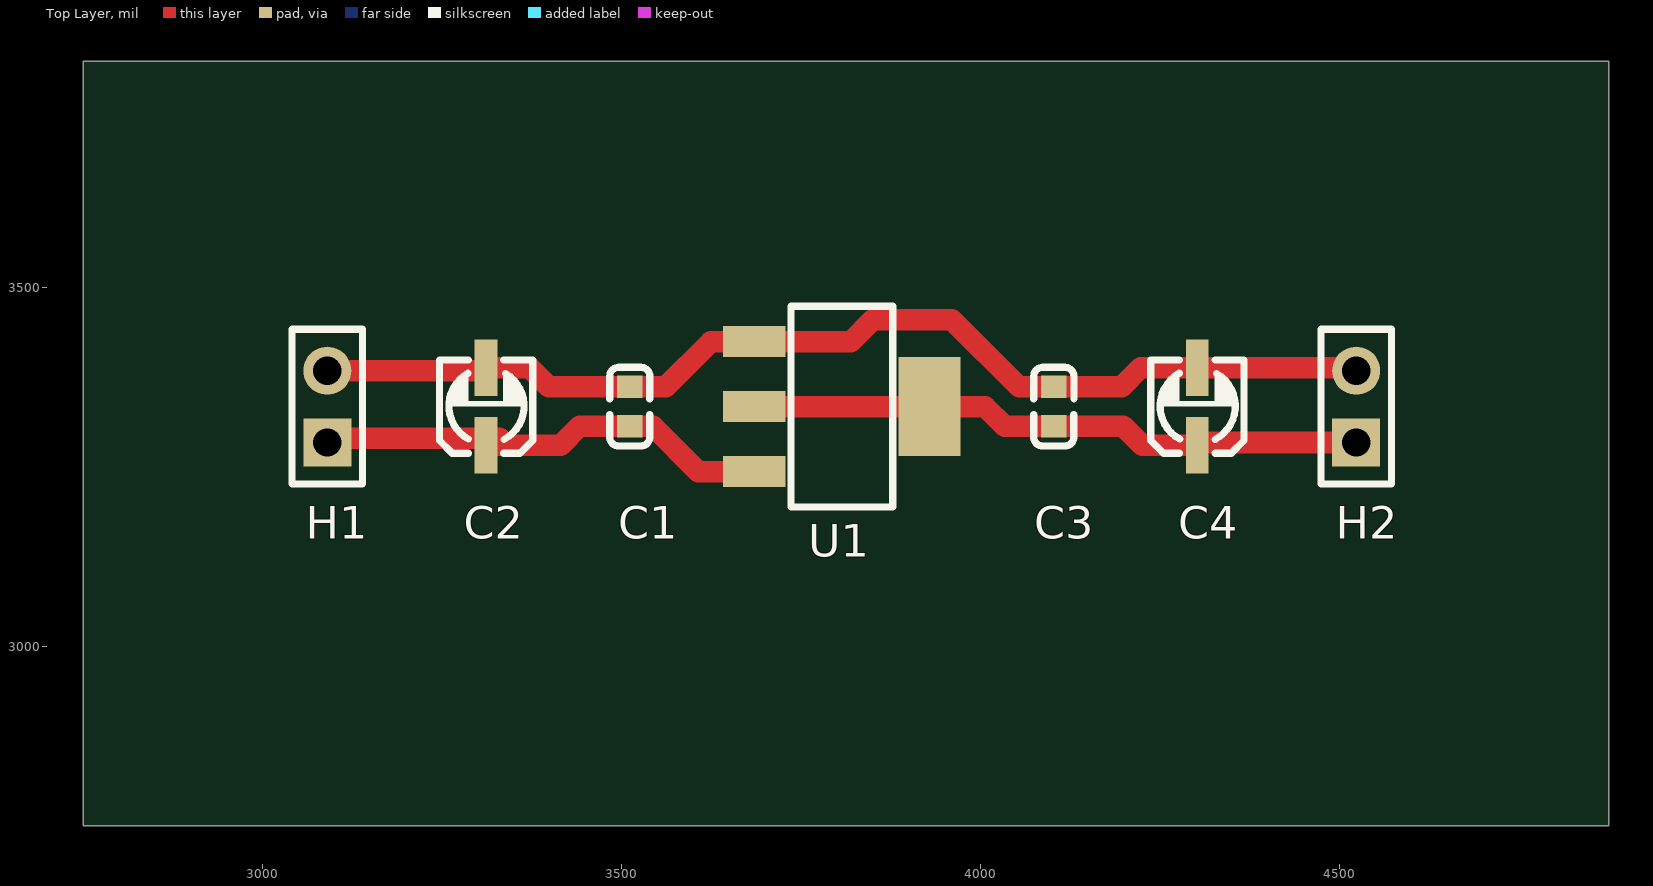
[diagram p0: Top Layer view]
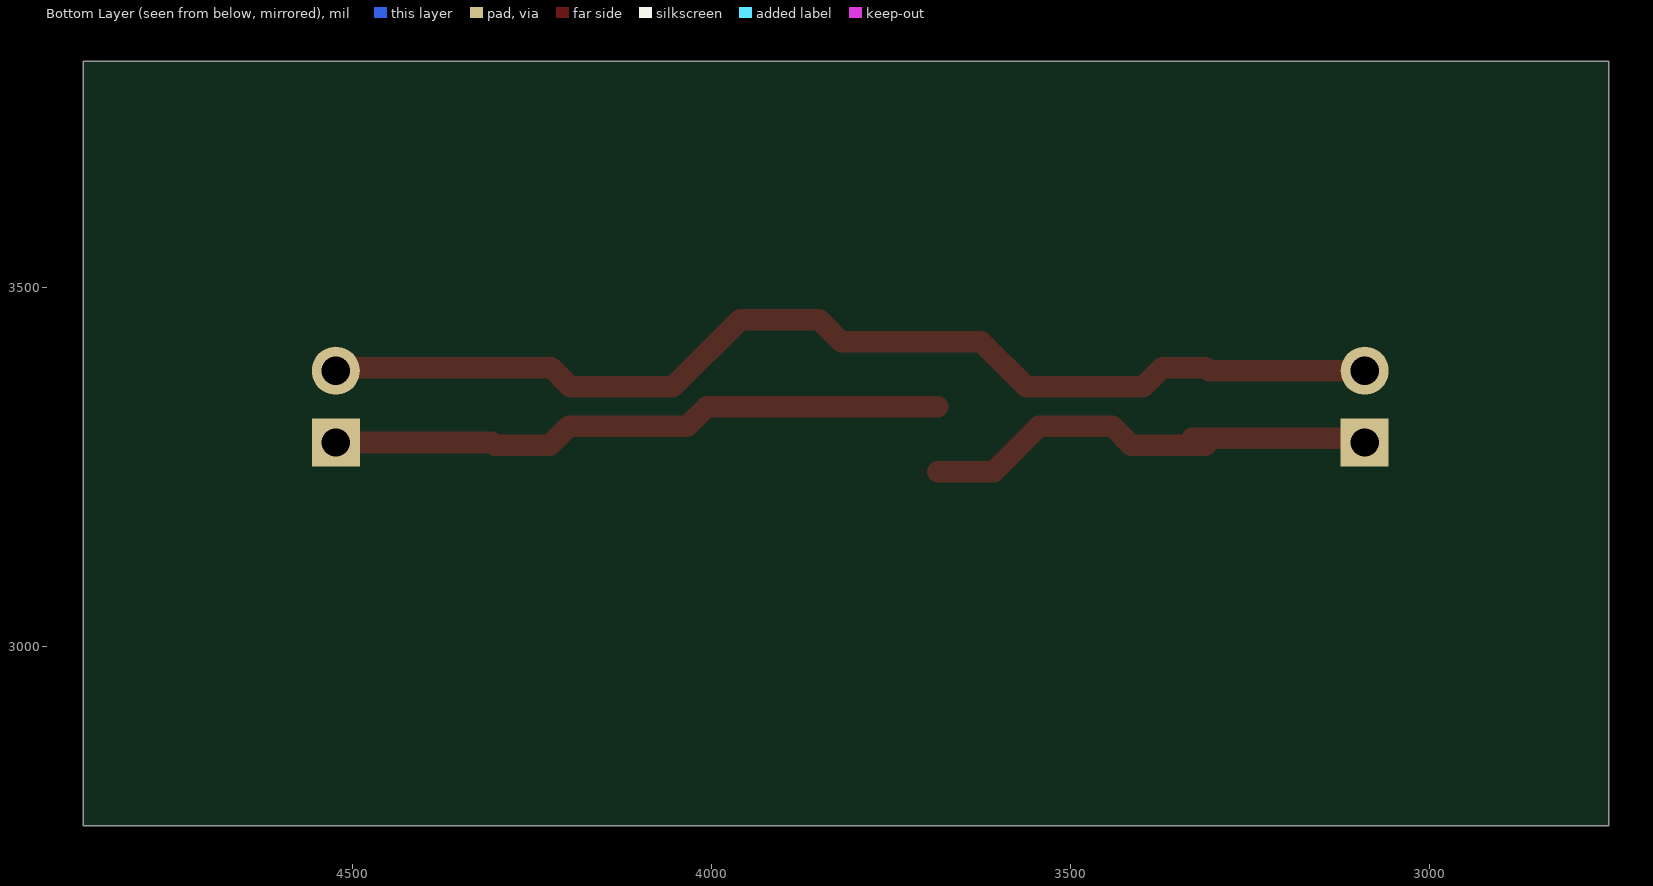
[diagram p1: Bottom Layer view, seen from below]
# Altium PCB MISC52016.pcbdoc
Units mil, origin at the board's own origin, x right, y up, seen from the top; angles counter-clockwise.
Board outline 2125 x 1065 mil, 2 copper layers (Top Layer, Bottom Layer), stack 62.206 mil thick; 7 components, 3 nets, 16 pads, 0 vias.

## Layer stack, top to bottom
Top Solder Mask Layer: solder mask 0.394, Dk 3.3
Top Layer: signal copper 1.379
Dielectric1: surface 59.449, FR4, Dk 4.5
Bottom Layer: signal copper 1.378
Bottom Solder Mask Layer: solder mask 0.394, Dk 3.3

## Board outline
4875,2750 2750,2750 2750,3815 4875,3815

## Design rules (kind name [scope] priority, off if disabled: settings)
BoardOutlineClearance copperThickness2oz_1 [All] p2 off: genericclearance=7.99 ignorepadtopadclearanceinfootprint=FALSE except(0: Arc-SplitContinuation Track-SplitContinuation SMDPad-SplitContinuation THPad-SplitContinuation Via-SplitContinuation Fill-SplitContinuation Region-SplitContinuation Poly-SplitContinuation Text-SplitContinuation Hole-SplitContinuation; 5.98: Arc-CutoutEdge SMDPad-CutoutEdge THPad-CutoutEdge Via-CutoutEdge Fill-CutoutEdge Region-CutoutEdge Text-CutoutEdge; 6.93: Hole-OutlineEdge Hole-CutoutEdge; 10: Poly-OutlineEdge Poly-CutoutEdge; 11.81: Arc-OutlineEdge Track-OutlineEdge SMDPad-OutlineEdge THPad-OutlineEdge Via-OutlineEdge Fill-OutlineEdge Region-OutlineEdge Text-OutlineEdge Track-CutoutEdge)
BoardOutlineClearance copperThickness1oz_1 [All] p4: genericclearance=4.02 ignorepadtopadclearanceinfootprint=FALSE except(0: Arc-SplitContinuation Track-SplitContinuation SMDPad-SplitContinuation THPad-SplitContinuation Via-SplitContinuation Fill-SplitContinuation Region-SplitContinuation Poly-SplitContinuation Text-SplitContinuation Hole-SplitContinuation; 6: SMDPad-CutoutEdge THPad-CutoutEdge Via-CutoutEdge Fill-CutoutEdge Region-CutoutEdge Text-CutoutEdge; 6.93: Hole-OutlineEdge Hole-CutoutEdge; 10: Poly-OutlineEdge Poly-CutoutEdge; 11.8: Arc-OutlineEdge Track-OutlineEdge SMDPad-OutlineEdge THPad-OutlineEdge Via-OutlineEdge Fill-OutlineEdge Region-OutlineEdge Text-OutlineEdge; 11.81: Arc-CutoutEdge Track-CutoutEdge)
Clearance copperThickness2oz [All] p1 off: gap=7.99 ignorepadtopadclearanceinfootprint=FALSE except(5.98: SMDPad-Track SMDPad-SMDPad THPad-Track SMDPad-THPad THPad-THPad Track-Via SMDPad-Via THPad-Via Via-Via Fill-Track Region-Track Fill-SMDPad Region-SMDPad Fill-THPad Region-THPad Fill-Via Region-Via Fill-Fill Fill-Region Region-Region Arc-Track Arc-SMDPad Arc-THPad Arc-Via Fill-Arc Region-Arc Arc-Arc Text-Track SMDPad-Text Text-THPad Text-Via Fill-Text Region-Text Arc-Text Text-Text; 6.93: Hole-Track Hole-SMDPad Hole-THPad Hole-Via Fill-Hole Region-Hole Hole-Arc Hole-Text; 10: Poly-Track Poly-SMDPad Poly-THPad Poly-Via Poly-Fill Poly-Region Poly-Poly Poly-Arc Poly-Text Poly-Hole)
Clearance copperThickness1oz [All] p3: gap=4.02 ignorepadtopadclearanceinfootprint=FALSE except(5.98: SMDPad-Track SMDPad-SMDPad THPad-Track SMDPad-THPad THPad-THPad Track-Via SMDPad-Via THPad-Via Via-Via Fill-Track Region-Track Fill-SMDPad Region-SMDPad Fill-THPad Region-THPad Fill-Via Region-Via Fill-Fill Fill-Region Region-Region; 6: Arc-Track Arc-SMDPad Arc-THPad Arc-Via Fill-Arc Region-Arc Arc-Arc Text-Track SMDPad-Text Text-THPad Text-Via Fill-Text Region-Text Arc-Text Text-Text; 6.93: Hole-Track Hole-SMDPad Hole-THPad Hole-Via Fill-Hole Region-Hole Hole-Arc Hole-Text; 10: Poly-Track Poly-SMDPad Poly-THPad Poly-Via Poly-Fill Poly-Region Poly-Poly Poly-Arc Poly-Text Poly-Hole)
DiffPairsRouting differentialPair [All] p1: maxlimit=6 minlimit=6 mostfreqgap=6 toplayer_minwidth=5 toplayer_prefwidth=10 toplayer_maxwidth=100 toplayer_mingap=6 toplayer_prefgap=6 toplayer_maxgap=6 bottomlayer_minwidth=5 bottomlayer_prefwidth=10 bottomlayer_maxwidth=100 bottomlayer_mingap=6 bottomlayer_prefgap=6 bottomlayer_maxgap=6 maxuncoupledlength=10
HoleToHoleClearance otherClearance [All] p1: gap=11.81 allowstackedmicrovias=TRUE
Length netLength [All] p1: minlimit=0 maxlimit=0
MatchedLengths netLengthTolerance [All] p1: tolerance=1000
PasteMaskExpansion pasteMaskExpansion [All] p1: expansion=0
PlaneConnect innerPlane [All] p1: planeconnectstyle=Relief reliefexpansion=20 reliefentries=4 reliefconductorwidth=10 reliefairgap=10
PolygonConnect copperRegion [All] p1: connectstyle=Relief reliefconductorwidth=10 reliefentries=4 polygonreliefangle="90 Angle" airgapwidth=10 via.connectstyle=Relief via.reliefconductorwidth=10 via.reliefentries=4 via.polygonreliefangle="90 Angle" via.airgapwidth=10
RoutingVias viaSize [All] p1: holewidth=12.01 width=24.02 viastyle="Through Hole" minholewidth=11.81 minwidth=19.68 maxholewidth=248.03 maxwidth=393.7
SolderMaskExpansion solderMaskExpansion [IsVia] p1: expansion=-1000 istentingtop=TRUE
SolderMaskExpansion solderMaskExpansion [All] p2: expansion=2 istentingtop=FALSE
Width copperThickness2oz_2 [All] p1 off: maxlimit=100 minlimit=8 preferedwidth=10
Width copperThickness1oz_2 [All] p2: maxlimit=100 minlimit=5 preferedwidth=10

## Components (designator, comment, footprint, x,y, rotation, side; value= is the part's Value field where it differs from the comment)
C1 "100nF" C0603 3511.29,3333.9 r270 top
C2 "10uF" C_Ele_SMD_3x5.4mm 3311.63,3334.1 r270 top
C3 "100nF" C0603 4101.93,3333.9 r270 top
C4 "10uF" C_Ele_SMD_3x5.4mm 4302.3,3334.1 r270 top
H1 "" HDR-TH_2P-P2.54-V-F 3090,3333.9 r90 top
H2 "" HDR-TH_2P-P2.54-V-F 4523.22,3333.9 r90 top
U1 "" SOT_223 3807.67,3333.9 r270 top

## Footprints (in the part's own frame and the unit in brackets; to place one, negate y for a bottom-side part, rotate by r counter-clockwise, add the part's x,y. Pads: shape width x height; smd on the part's side, far side on the other; paste and mask are expansions set on the pad)
C0603 [mm]
  rect 0.8x0.9 smd: 1(-0.7,0) 2(0.7,0)
  silkscreen extent -1.39,-0.71 1.39,0.71
C_Ele_SMD_3x5.4mm [mil]
  rect 78.7x31.5 smd paste+0 mask+2: 1(54.1,-0.55) 2(-53.7,-0.55)
  silkscreen extent -65,-65 65,65
HDR-TH_2P-P2.54-V-F [mm]
  rect 1.7x1.7 hole 1: 1(-1.27,0)
  round 1.7 hole 1: 2(1.27,0)
  silkscreen extent -2.74,-1.25 2.74,1.25
SOT_223 [mil]
  rect 43.3x86.6 smd paste+0 mask+2: 1(-90.5,-123.05) 2(0,-123.05) 3(90.6,-123.05)
  rect 137.8x86.6 smd paste+0 mask+2: 4(0,120.95)
  silkscreen extent -140,-72 140,70

## Nets (pads, with @x,y where several pads share a name; then routed paths per layer and width w, separated by ;. In a path a pad name is that pad's centre, name@x,y a point inside that pad or via, vN(x,y) a via of type N, cw(c..) or ccw(c..) an arc to the next point about the centre after c; other vN are vias at no path point)
+5V: C1.2 C2.1 H1.1 U1.3 | length 653.1
  Top Layer w30: H1.1 3096.1,3290 3330,3290 ; C2.1 3415,3280 3441.34,3306.34 C1.2 3543.66,3306.34 3606.7,3243.3 U1.3
GND: C1.1 C2.2 C3.1 C4.2 H1.2 H2.2 U1.1 | length 1535.8
  Top Layer w30: H1.2 3307.18,3383.9 C2.2 3372.2,3387.8 3398.54,3361.46 C1.1 3561.46,3361.46 3624.4,3424.4 U1.1 3819.4,3424.4 3850,3455 3960,3455 4053.54,3361.46 C3.1 4196.46,3361.46 4222.8,3387.8 C4.2 4519.32,3387.8 H2.2
VCC: C3.2 C4.1 H2.1 U1.2 U1.4 | length 862.6
  Top Layer w30: U1.2 U1.4 4006.1,3333.9 4033.66,3306.34 C3.2 4198.66,3306.34 4225,3280 C4.1 4305.65,3283.9 H2.1

## Silkscreen, mask and mechanical layers (free items; w line width, h text height)
Mechanical Layer:
  lines w10: 3000,3000 3000,3565 4625,3565 4625,3000 3000,3000